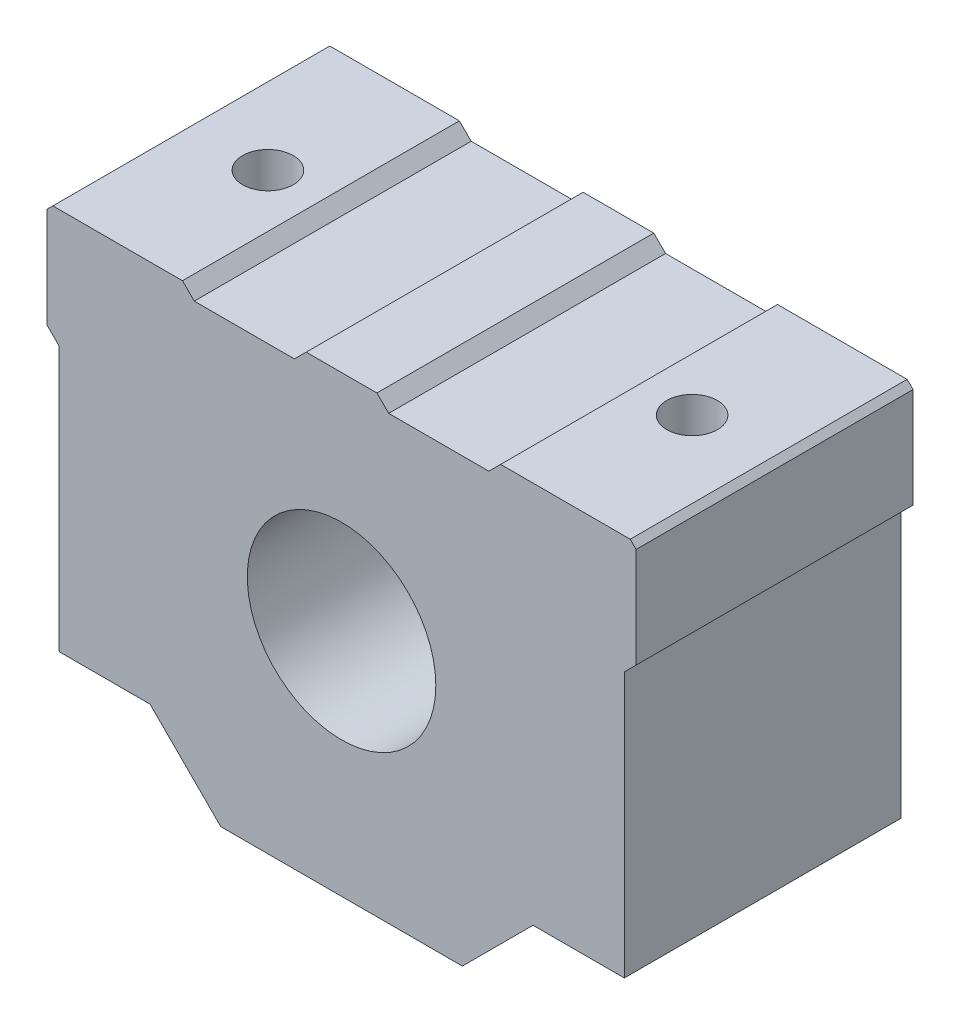
from build123d import *

# Parameters (mm, degrees)
SKETCH_1_R          = 8
EXTRUDE_1_DEPTH     = 23.5
SKETCH_2_R          = 2.15
CUT_EXTRUDE_1_DEPTH = 52.570340313


with BuildPart() as part:
    # 草图1 → 凸台-拉伸1 (new body)
    with BuildSketch(Plane.XY):
        Polygon((-10.25, -19.5), (10.25, -19.5), (16.25, -13.5), (24, -13.5), (24, 9), (25, 10), (25, 18.5), (24.5, 19), (13.5, 19), (12.5, 18), (4, 18), (3, 19), (-3, 19), (-4, 18), (-12.5, 18), (-13.5, 19), (-24.5, 19), (-25, 18.5), (-25, 10), (-24, 9), (-24, -13.5), (-16.25, -13.5), align=None)
        Circle(SKETCH_1_R, mode=Mode.SUBTRACT)
    extrude(amount=EXTRUDE_1_DEPTH)

    # 草图2 → 切除-拉伸1 (cut, through all)
    with BuildSketch(Plane(origin=(0, 19, 0), x_dir=(1, 0, 0), z_dir=(0, 1, 0))):
        with Locations(Location((-18, -11.75, 0), (0, 0, 270))):
            Circle(SKETCH_2_R)
        with Locations(Location((18, -11.75, 0), (0, 0, 270))):
            Circle(SKETCH_2_R)
    extrude(amount=-CUT_EXTRUDE_1_DEPTH, mode=Mode.SUBTRACT)


solid = part.part
